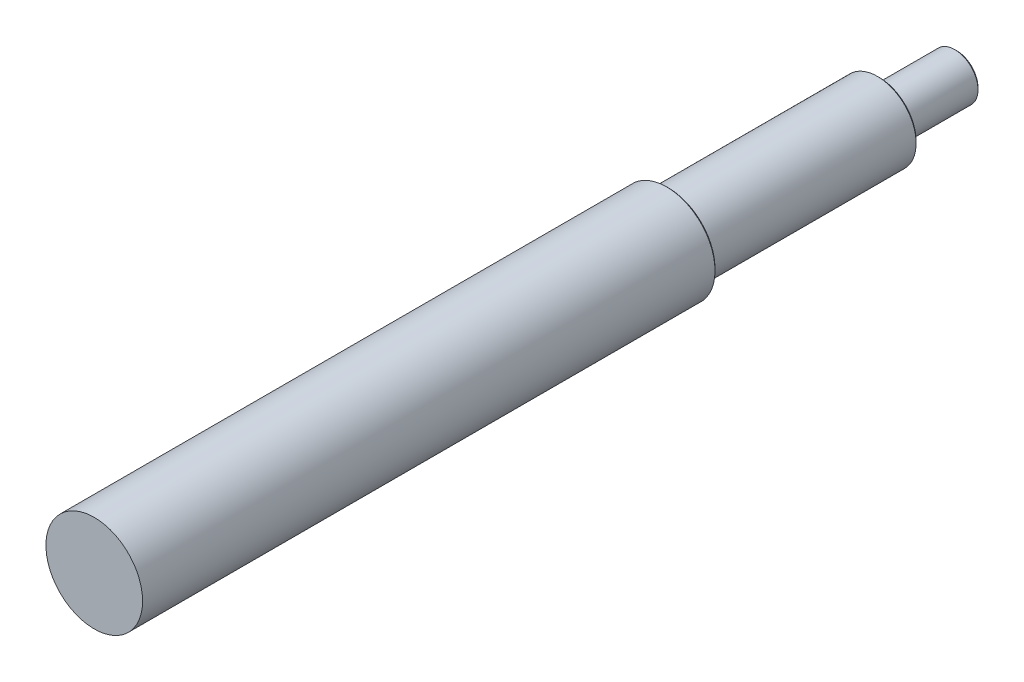
from build123d import *

# Parameters (mm, degrees)
EXTRUDE_1_DEPTH      = 100
EXTRUDE_1_DEPTH_BACK = 346
SKETCH_1_R           = 25
SKETCH_2_R           = 25
SKETCH_2_R_2         = 20
CUT_EXTRUDE_1_DEPTH  = 109
SKETCH_3_R           = 25
SKETCH_3_R_2         = 12
CUT_EXTRUDE_2_DEPTH  = 40
CHAMFER_1_SIZE       = 1


with BuildPart() as part:
    # 草图1 → 凸台-拉伸1 (new, two sides: drawn at the far end of the back side and taken through both)
    with BuildSketch(Plane.XY.offset(-EXTRUDE_1_DEPTH_BACK)):
        Circle(SKETCH_1_R)
    extrude(amount=EXTRUDE_1_DEPTH + EXTRUDE_1_DEPTH_BACK)

    # 草图2 → 切除-拉伸1 (cut)
    with BuildSketch(Plane(origin=(0, 0, -306), x_dir=(-1, 0, 0), z_dir=(0, 0, -1))):
        with Locations(Location((0, 0, 0), (0, 0, 180))):
            Circle(SKETCH_2_R)
        Circle(SKETCH_2_R_2, mode=Mode.SUBTRACT)
    extrude(amount=-CUT_EXTRUDE_1_DEPTH, mode=Mode.SUBTRACT)

    # 草图3 → 切除-拉伸2 (cut)
    with BuildSketch(Plane(origin=(0, 0, -346), x_dir=(-1, 0, 0), z_dir=(0, 0, -1))):
        with Locations(Location((0, 0, 0), (0, 0, 180))):
            Circle(SKETCH_3_R)
        Circle(SKETCH_3_R_2, mode=Mode.SUBTRACT)
    extrude(amount=-CUT_EXTRUDE_2_DEPTH, mode=Mode.SUBTRACT)

    # 倒角1
    chamfer_1_edges = [part.edges().sort_by_distance(p)[0] for p in [
        (20, 0, -306),
        (12, 0, -346),
        (-25, 0, -197),
    ]]
    chamfer(chamfer_1_edges, length=CHAMFER_1_SIZE)


solid = part.part
